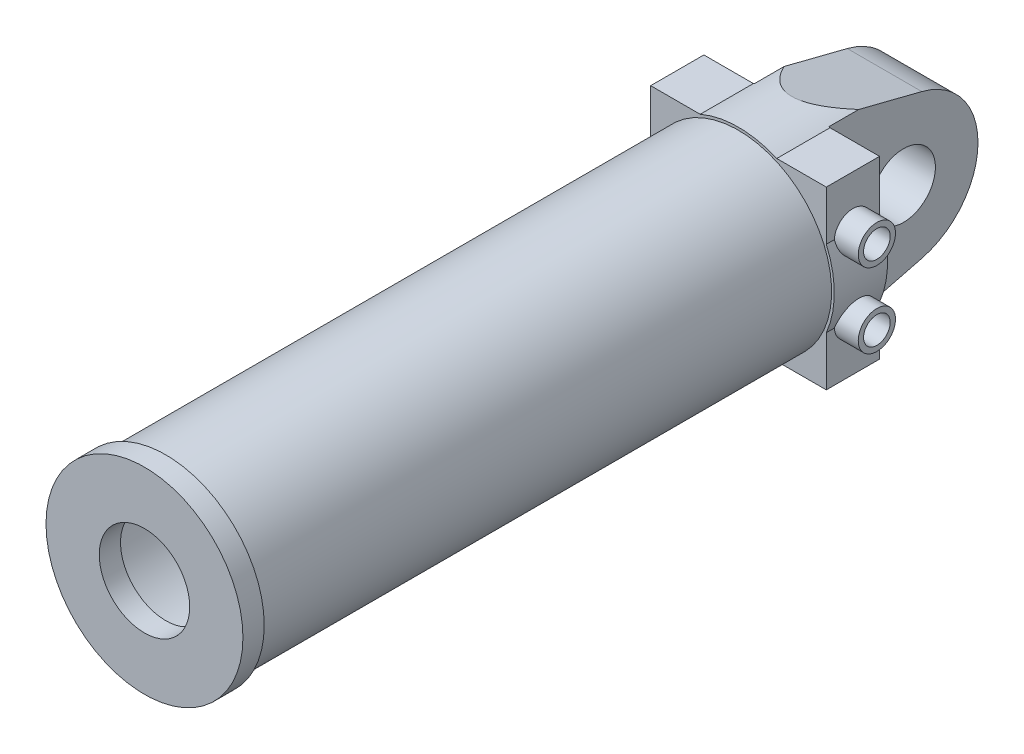
from build123d import *

# Parameters (mm, degrees)
SKETCH_1_R          = 87.5
SKETCH_1_R_2        = 77.5
EXTRUDE_1_DEPTH     = 558
SKETCH_4_R          = 90
EXTRUDE_2_DEPTH     = 50
SKETCH_5_R          = 30
EXTRUDE_3_DEPTH     = 35
SKETCH_6_OUTSIDE_W  = 340.026
SKETCH_6_OUTSIDE_H  = 340.026
SKETCH_6_OUTSIDE_R  = 90
CUT_EXTRUDE_2_DEPTH = 622.179523165
SKETCH_7_R          = 17.5
SKETCH_7_R_2        = 12.5
EXTRUDE_4_DEPTH     = 105
SKETCH_8_R          = 92.5
SKETCH_8_R_2        = 42.5
EXTRUDE_5_DEPTH     = 20
SKETCH_9_W          = 165
SKETCH_9_H          = 165
EXTRUDE_6_DEPTH     = 50


with BuildPart() as part:
    # 草图1 → 凸台-拉伸1 (new body)
    with BuildSketch(Plane.XY):
        Circle(SKETCH_1_R)
        Circle(SKETCH_1_R_2, mode=Mode.SUBTRACT)
    extrude(amount=EXTRUDE_1_DEPTH)

    # 草图4 → 凸台-拉伸2 (add)
    with BuildSketch(Plane(origin=(0, 0, 0), x_dir=(-1, 0, 0), z_dir=(0, 0, -1))):
        Circle(SKETCH_4_R)
    extrude(amount=EXTRUDE_2_DEPTH)

    # 草图5 → 凸台-拉伸3 (add, symmetric)
    with BuildSketch(Plane(origin=(0, 0, 0), x_dir=(0, 0, -1), z_dir=(1, 0, 0))):
        with BuildLine():
            Line((50, 90), (137.230769231, 67.846153846))
            ThreePointArc((137.230769231, 67.846153846), (190, 0), (137.230769231, -67.846153846))
            Line((137.230769231, -67.846153846), (50, -90))
            Line((50, -90), (50, 90))
        make_face()
        with Locations((120, 0)):
            Circle(SKETCH_5_R, mode=Mode.SUBTRACT)
    extrude(amount=EXTRUDE_3_DEPTH, both=True)

    # 草图6 outside → 切除-拉伸2 (cut, through all)
    with BuildSketch(Plane(origin=(0, 0, -50), x_dir=(-1, 0, 0), z_dir=(0, 0, -1))):
        Rectangle(SKETCH_6_OUTSIDE_W, SKETCH_6_OUTSIDE_H)
        with Locations(Location((0, 0, 0), (0, 0, 247.114619524))):
            Circle(SKETCH_6_OUTSIDE_R, mode=Mode.SUBTRACT)
    extrude(amount=CUT_EXTRUDE_2_DEPTH, mode=Mode.SUBTRACT)

    # 草图7 → 凸台-拉伸4 (add)
    # profile 1 of 2: a face of its own
    with BuildSketch(Plane(origin=(0, 0, 0), x_dir=(0, 0, -1), z_dir=(1, 0, 0))):
        with Locations(Location((25, 35, 0), (0, 0, 180))):
            Circle(SKETCH_7_R)
        with Locations(Location((25, 35, 0), (0, 0, 180))):
            Circle(SKETCH_7_R_2, mode=Mode.SUBTRACT)
    # profile 2 of 2: a face of its own
    with BuildSketch(Plane(origin=(0, 0, 0), x_dir=(0, 0, -1), z_dir=(1, 0, 0))):
        with Locations(Location((25, -35, 0), (0, 0, 180))):
            Circle(SKETCH_7_R)
        with Locations(Location((25, -35, 0), (0, 0, 180))):
            Circle(SKETCH_7_R_2, mode=Mode.SUBTRACT)
    extrude(amount=EXTRUDE_4_DEPTH)

    # 草图8 → 凸台-拉伸5 (add)
    with BuildSketch(Plane.XY.offset(558)):
        Circle(SKETCH_8_R)
        Circle(SKETCH_8_R_2, mode=Mode.SUBTRACT)
    extrude(amount=-EXTRUDE_5_DEPTH)

    # 草图9 → 凸台-拉伸6 (add)
    with BuildSketch(Plane(origin=(0, 0, -50), x_dir=(-1, 0, 0), z_dir=(0, 0, -1))):
        Rectangle(SKETCH_9_W, SKETCH_9_H)
    extrude(amount=-EXTRUDE_6_DEPTH)


solid = part.part
